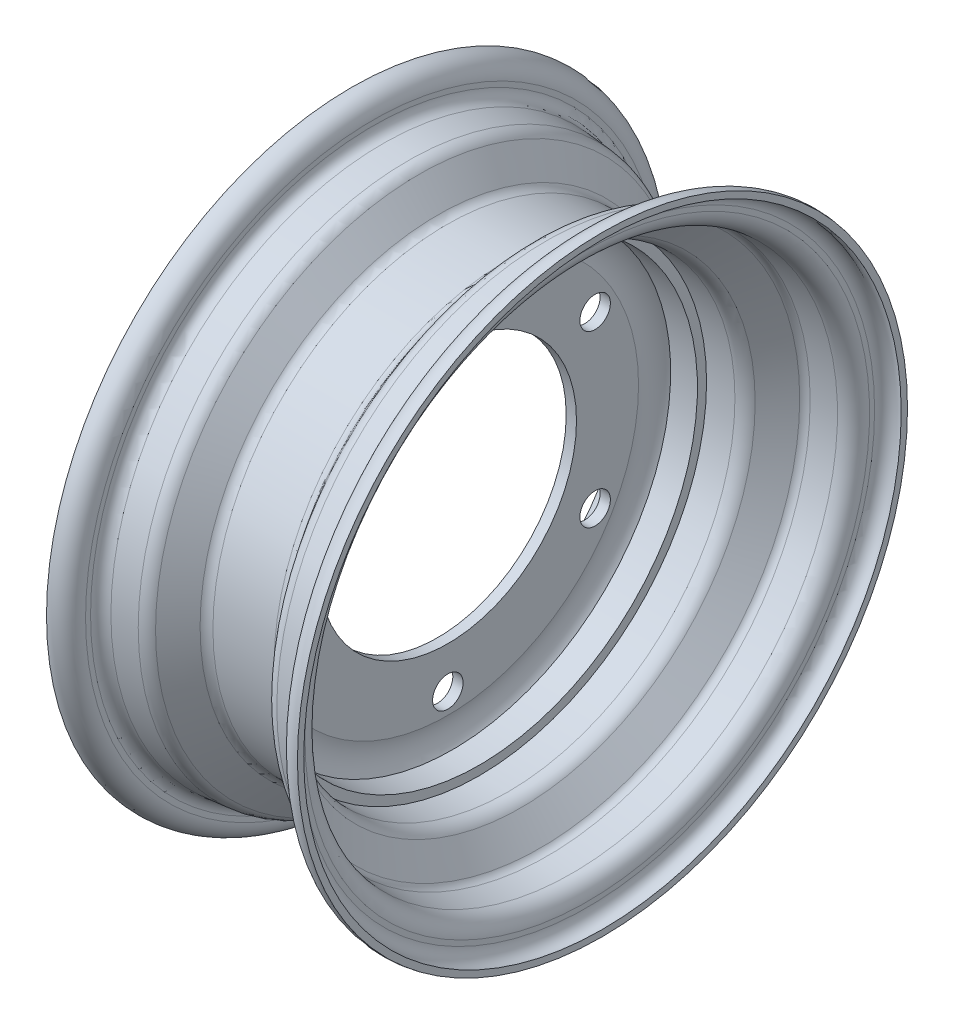
SolidWorks part; units mm, degrees
material "7079 合金"
ref_plane "前视基准面" through (0, 0, 0) normal (0, 0, 1) x (1, 0, 0)
ref_plane "上视基准面" through (0, 0, 0) normal (0, 1, 0) x (1, 0, 0)
ref_plane "右视基准面" through (0, 0, 0) normal (1, 0, 0) x (0, 0, -1)
sketch "草图1" plane through (0, 0, 0) normal (0, 0, 1) x (1, 0, 0)
  line L23 (84.4803, 317.7627) -> (83.8413, 320.3941)
  line L26 (96.4554, 268.4534) -> (84.4803, 317.7627)
  line L27 (97.0221, 268.0882) -> (96.9199, 268.0882)
  line L28 (97.5, 244.8015) -> (97.5, 267.6103)
  line L29 (96.8899, 244.3235) -> (97.0221, 244.3235)
  line L30 (78.5236, 193.1098) -> (96.4391, 244.0043)
  line L31 (79.1815, 192.6755) -> (78.6405, 192.866)
  line L32 (79.1079, 191.8907) -> (79.2983, 192.4317)
  line L33 (78.3231, 191.9643) -> (78.8641, 191.7739)
  line L34 (77.0954, 189.0523) -> (78.0793, 191.8475)
  line L35 (77.7532, 188.6181) -> (77.2122, 188.8085)
  line L36 (77.6796, 187.8333) -> (77.8701, 188.3743)
  line L37 (76.8948, 187.9069) -> (77.4358, 187.7165)
  line L38 (75.6671, 184.9949) -> (76.651, 187.79)
  line L39 (76.325, 184.5607) -> (75.784, 184.7511)
  line L40 (76.2514, 183.7759) -> (76.4418, 184.3169)
  line L41 (75.4666, 183.8495) -> (76.0076, 183.659)
  line L42 (73.1324, 177.7941) -> (75.2228, 183.7326)
  line L43 (59.75, 177.7941) -> (73.1324, 177.7941)
  line L44 (59.75, 162.5) -> (59.75, 177.7941)
  line L45 (50.25, 162.5) -> (59.75, 162.5)
  line L46 (50.25, 187.3529) -> (50.25, 162.5)
  line L47 (66.4222, 187.3529) -> (50.25, 187.3529)
  line L48 (88.0074, 248.6723) -> (66.4222, 187.3529)
  line L49 (88.0074, 263.1405) -> (88.0074, 248.6723)
  line L50 (75.7794, 313.4968) -> (88.0074, 263.1405)
  line L51 (-66.4905, 320.8) -> (66.4905, 320.8)
  line L52 (-88.0074, 263.1405) -> (-75.7794, 313.4968)
  line L53 (-88.0074, 248.6723) -> (-88.0074, 263.1405)
  line L54 (-66.4222, 187.3529) -> (-88.0074, 248.6723)
  line L55 (-50.25, 187.3529) -> (-66.4222, 187.3529)
  line L56 (-50.25, 162.5) -> (-50.25, 187.3529)
  line L57 (-59.75, 162.5) -> (-50.25, 162.5)
  line L58 (-59.75, 177.7941) -> (-59.75, 162.5)
  line L59 (-73.1324, 177.7941) -> (-59.75, 177.7941)
  line L60 (-75.2228, 183.7326) -> (-73.1324, 177.7941)
  line L61 (-76.0076, 183.659) -> (-75.4666, 183.8495)
  line L62 (-76.4418, 184.3169) -> (-76.2514, 183.7759)
  line L63 (-75.784, 184.7511) -> (-76.325, 184.5607)
  line L64 (-76.651, 187.79) -> (-75.6671, 184.9949)
  line L65 (-77.4358, 187.7165) -> (-76.8948, 187.9069)
  line L66 (-77.8701, 188.3743) -> (-77.6796, 187.8333)
  line L67 (-77.2122, 188.8085) -> (-77.7532, 188.6181)
  line L68 (-78.0793, 191.8475) -> (-77.0954, 189.0523)
  line L69 (-78.8641, 191.7739) -> (-78.3231, 191.9643)
  line L70 (-79.2983, 192.4317) -> (-79.1079, 191.8907)
  line L71 (-78.6405, 192.866) -> (-79.1815, 192.6755)
  line L72 (-96.4391, 244.0043) -> (-78.5236, 193.1098)
  line L73 (-97.0221, 244.3235) -> (-96.8899, 244.3235)
  line L74 (-97.5, 267.6103) -> (-97.5, 244.8015)
  line L75 (-96.9199, 268.0882) -> (-97.0221, 268.0882)
  line L76 (-83.8413, 320.3941) -> (-96.4554, 268.4534)
  line L80 (0, 0) -> (0, 335) construction
  line L81 (-50.25, 162.5) -> (50.25, 162.5) construction
  line L82 (0, 0) -> (328.2798, 0) construction
  line L83 (-65.2636, 335) -> (65.2636, 335)
  arc A1 (-65.2636, 335) -> (-83.8413, 320.3941) centre (-65.2636, 315.8824) ccw
  arc A2 (83.8413, 320.3941) -> (65.2636, 335) centre (65.2636, 315.8824) ccw
  arc A10 (96.4554, 268.4534) -> (96.9199, 268.0882) centre (96.9199, 268.5662) ccw
  arc A11 (97.5, 267.6103) -> (97.0221, 268.0882) centre (97.0221, 267.6103) ccw
  arc A12 (97.0221, 244.3235) -> (97.5, 244.8015) centre (97.0221, 244.8015) ccw
  arc A13 (96.8899, 244.3235) -> (96.4391, 244.0043) centre (96.8899, 243.8456) ccw
  arc A14 (78.5236, 193.1098) -> (78.6405, 192.866) centre (78.704, 193.0463) ccw
  arc A15 (79.2983, 192.4317) -> (79.1815, 192.6755) centre (79.118, 192.4952) ccw
  arc A16 (78.8641, 191.7739) -> (79.1079, 191.8907) centre (78.9276, 191.9542) ccw
  arc A17 (78.3231, 191.9643) -> (78.0793, 191.8475) centre (78.2596, 191.784) ccw
  arc A18 (77.0954, 189.0523) -> (77.2122, 188.8085) centre (77.2757, 188.9889) ccw
  arc A19 (77.8701, 188.3743) -> (77.7532, 188.6181) centre (77.6897, 188.4378) ccw
  arc A20 (77.4358, 187.7165) -> (77.6796, 187.8333) centre (77.4993, 187.8968) ccw
  arc A21 (76.8948, 187.9069) -> (76.651, 187.79) centre (76.8314, 187.7266) ccw
  arc A22 (75.6671, 184.9949) -> (75.784, 184.7511) centre (75.8474, 184.9314) ccw
  arc A23 (76.4418, 184.3169) -> (76.325, 184.5607) centre (76.2615, 184.3803) ccw
  arc A24 (76.0076, 183.659) -> (76.2514, 183.7759) centre (76.071, 183.8394) ccw
  arc A25 (75.4666, 183.8495) -> (75.2228, 183.7326) centre (75.4031, 183.6691) ccw
  arc A26 (75.7794, 313.4968) -> (66.4905, 320.8) centre (66.4905, 311.2412) ccw
  arc A27 (-66.4905, 320.8) -> (-75.7794, 313.4968) centre (-66.4905, 311.2412) ccw
  arc A28 (-75.2228, 183.7326) -> (-75.4666, 183.8495) centre (-75.4031, 183.6691) ccw
  arc A29 (-76.2514, 183.7759) -> (-76.0076, 183.659) centre (-76.071, 183.8394) ccw
  arc A30 (-76.325, 184.5607) -> (-76.4418, 184.3169) centre (-76.2615, 184.3803) ccw
  arc A31 (-75.784, 184.7511) -> (-75.6671, 184.9949) centre (-75.8474, 184.9314) ccw
  arc A32 (-76.651, 187.79) -> (-76.8948, 187.9069) centre (-76.8314, 187.7266) ccw
  arc A33 (-77.6796, 187.8333) -> (-77.4358, 187.7165) centre (-77.4993, 187.8968) ccw
  arc A34 (-77.7532, 188.6181) -> (-77.8701, 188.3743) centre (-77.6897, 188.4378) ccw
  arc A35 (-77.2122, 188.8085) -> (-77.0954, 189.0523) centre (-77.2757, 188.9889) ccw
  arc A36 (-78.0793, 191.8475) -> (-78.3231, 191.9643) centre (-78.2596, 191.784) ccw
  arc A37 (-79.1079, 191.8907) -> (-78.8641, 191.7739) centre (-78.9276, 191.9542) ccw
  arc A38 (-79.1815, 192.6755) -> (-79.2983, 192.4317) centre (-79.118, 192.4952) ccw
  arc A39 (-78.6405, 192.866) -> (-78.5236, 193.1098) centre (-78.704, 193.0463) ccw
  arc A40 (-96.4391, 244.0043) -> (-96.8899, 244.3235) centre (-96.8899, 243.8456) ccw
  arc A41 (-97.5, 244.8015) -> (-97.0221, 244.3235) centre (-97.0221, 244.8015) ccw
  arc A42 (-97.0221, 268.0882) -> (-97.5, 267.6103) centre (-97.0221, 267.6103) ccw
  arc A43 (-96.9199, 268.0882) -> (-96.4554, 268.4534) centre (-96.9199, 268.5662) ccw
  dimension "D2" = 14.2
  dimension "D3" = 0.4779
  dimension "D4" = 0.1912
  dimension "D5" = 9.5588
  dimension "D1" = 670
  dimension "D6" = 325
  dimension "D7" = 195
  dimension "D8" = 119.5
  dimension "D9" = 9.5
  dimension "D10" = 24.8529
  dimension "D11" = 15.2941
  dimension "D12" = 146.2647
sketch "草图2" plane through (0, 0, 0) normal (0, 0, 1) x (1, 0, 0)
  line L0 (55.0334, 158.3536) -> (40.3872, 157.0722)
  line L1 (60.7057, 167.4531) -> (60.7057, 164.5438)
  line L2 (73.1324, 174.1159) -> (73.1324, 177.7941)
  line L3 (64.2904, 164.5438) -> (64.2904, 167.4531)
  line L4 (40.6996, 153.5011) -> (55.3459, 154.7825)
  line L5 (25.683, 136.4516) -> (36.7734, 151.3128)
  line L6 (1.3, 132.5134) -> (17.8301, 132.5134)
  line L7 (1.3, 127.1981) -> (1.3, 132.5134)
  line L8 (-14.3052, 127.1981) -> (1.3, 127.1981)
  line L9 (-17, 75) -> (-17, 111.1619)
  line L10 (-23, 75) -> (-17, 75)
  line L11 (-23, 111.1619) -> (-23, 75)
  line L12 (-36.7734, 151.3128) -> (-25.683, 136.4516)
  line L13 (-55.3459, 154.7825) -> (-40.6996, 153.5011)
  line L14 (-64.2904, 167.4531) -> (-64.2904, 164.5438)
  line L15 (-73.1324, 177.7941) -> (-73.1324, 174.1159)
  line L16 (-60.7057, 164.5438) -> (-60.7057, 167.4531)
  line L17 (-40.3872, 157.0722) -> (-55.0334, 158.3536)
  line L18 (-22.8101, 138.5956) -> (-33.9004, 153.4568)
  line L19 (17.8301, 136.0981) -> (-17.8301, 136.0981)
  line L20 (33.9004, 153.4568) -> (22.8101, 138.5956)
  line L21 (-73.1324, 175.955) -> (73.1324, 175.955) construction
  line L22 (0, 175.955) -> (0, 175.971) construction
  line L23 (0, 0) -> (328.2798, 0) construction
  line L24 (0, 0) -> (0, 335) construction
  line L25 (0, 0) -> (328.2798, 0) construction
  line L26 (0, 0) -> (0, 335) construction
  line L28 (-26.6192, 105.5) -> (-19.2091, 105.5) construction
  line L29 (-26.6192, 105.5) -> (-26.6192, 94.5) construction
  line L30 (-26.6192, 94.5) -> (-19.2091, 94.5) construction
  line L31 (-19.2091, 105.5) -> (-19.2091, 94.5) construction
  arc A0 (40.3872, 157.0722) -> (33.9004, 153.4568) centre (41.1787, 148.0253) ccw
  arc A1 (55.0334, 158.3536) -> (60.7057, 164.5438) centre (54.4919, 164.5438) ccw
  arc A2 (73.1324, 177.7941) -> (60.7057, 167.4531) centre (71.2218, 167.4531) ccw
  arc A3 (73.1324, 174.1159) -> (64.2904, 167.4531) centre (71.2218, 167.4531) ccw
  arc A4 (55.3459, 154.7825) -> (64.2904, 164.5438) centre (54.4919, 164.5438) ccw
  arc A5 (40.6996, 153.5011) -> (36.7734, 151.3128) centre (41.1787, 148.0253) ccw
  arc A6 (17.8301, 132.5134) -> (25.683, 136.4516) centre (17.8301, 142.3119) ccw
  arc A10 (-23, 111.1619) -> (-23.7013, 115.2096) centre (-35.0314, 111.1619) ccw
  arc A13 (-25.683, 136.4516) -> (-17.8309, 132.5134) centre (-17.8301, 142.3119) ccw
  arc A14 (-36.7734, 151.3128) -> (-40.6996, 153.5011) centre (-41.1787, 148.0253) ccw
  arc A15 (-64.2904, 164.5438) -> (-55.3459, 154.7825) centre (-54.4919, 164.5438) ccw
  arc A16 (-64.2904, 167.4531) -> (-73.1324, 174.1159) centre (-71.2218, 167.4531) ccw
  arc A17 (-60.7057, 167.4531) -> (-73.1324, 177.7941) centre (-71.2218, 167.4531) ccw
  arc A18 (-60.7057, 164.5438) -> (-55.0334, 158.3536) centre (-54.4919, 164.5438) ccw
  arc A19 (-33.9004, 153.4568) -> (-40.3872, 157.0722) centre (-41.1787, 148.0253) ccw
  arc A20 (-22.8101, 138.5956) -> (-17.8301, 136.0981) centre (-17.8301, 142.3119) ccw
  arc A21 (17.8301, 136.0981) -> (22.8101, 138.5956) centre (17.8301, 142.3119) ccw
  arc A22 (-17.8309, 132.5134) -> (-23.7013, 115.2096) centre (-7.4158, 119.3323) ccw
  arc A23 (-14.3052, 127.1981) -> (-17, 111.1619) centre (0.5164, 116.4629) ccw
  point P0 (-0.029, 0.0006)
  point P19 (-19.2091, 100)
  dimension "D3" = 9.0815
  dimension "D4" = 6
  dimension "D5" = 8.9
  dimension "D6" = 2.6
  dimension "D7" = 11
  dimension "D8" = 34
  dimension "D9" = 200
  dimension "D2" = 150
revolve "旋转1" add sketch "草图2" angle 360 about L82
sketch "草图3" plane through (-23, 0, 0) normal (-1, 0, 0) x (0, 0, 1)
  line L0 (0, 0) -> (0, 335) construction
  circle A0 centre (0, 90) radius 6.5
  circle A1 centre (0, 0) radius 90 construction
  circle A2 centre (77.9423, 45) radius 6.5
  circle A3 centre (77.9423, -45) radius 6.5
  circle A4 centre (0, -90) radius 6.5
  circle A5 centre (-77.9423, -45) radius 6.5
  circle A6 centre (-77.9423, 45) radius 6.5
  point P18 (0, 0)
  dimension "D1" = 180
  dimension "D2" = 13
  dimension "D3" = 6
extrude "切除-拉伸1" [suppressed] cut sketch "草图3" against normal through all
scale "缩放比例1" scale about origin uniform scaling yes scale factor 0.731343
sketch "草图4" plane through (-16.8209, 0, 0) normal (-1, 0, 0) x (0, 0, 1)
  circle A0 centre (0, 0) radius 72.5 construction
  circle A1 centre (0, 72.5) radius 6.5
  circle A2 centre (62.7868, 36.25) radius 6.5
  circle A3 centre (62.7868, -36.25) radius 6.5
  circle A4 centre (0, -72.5) radius 6.5
  circle A5 centre (-62.7868, -36.25) radius 6.5
  circle A6 centre (-62.7868, 36.25) radius 6.5
  point P17 (0, 0)
  dimension "D1" = 145
  dimension "D2" = 13
  dimension "D3" = 6
extrude "切除-拉伸2" cut sketch "草图4" against normal up to next
